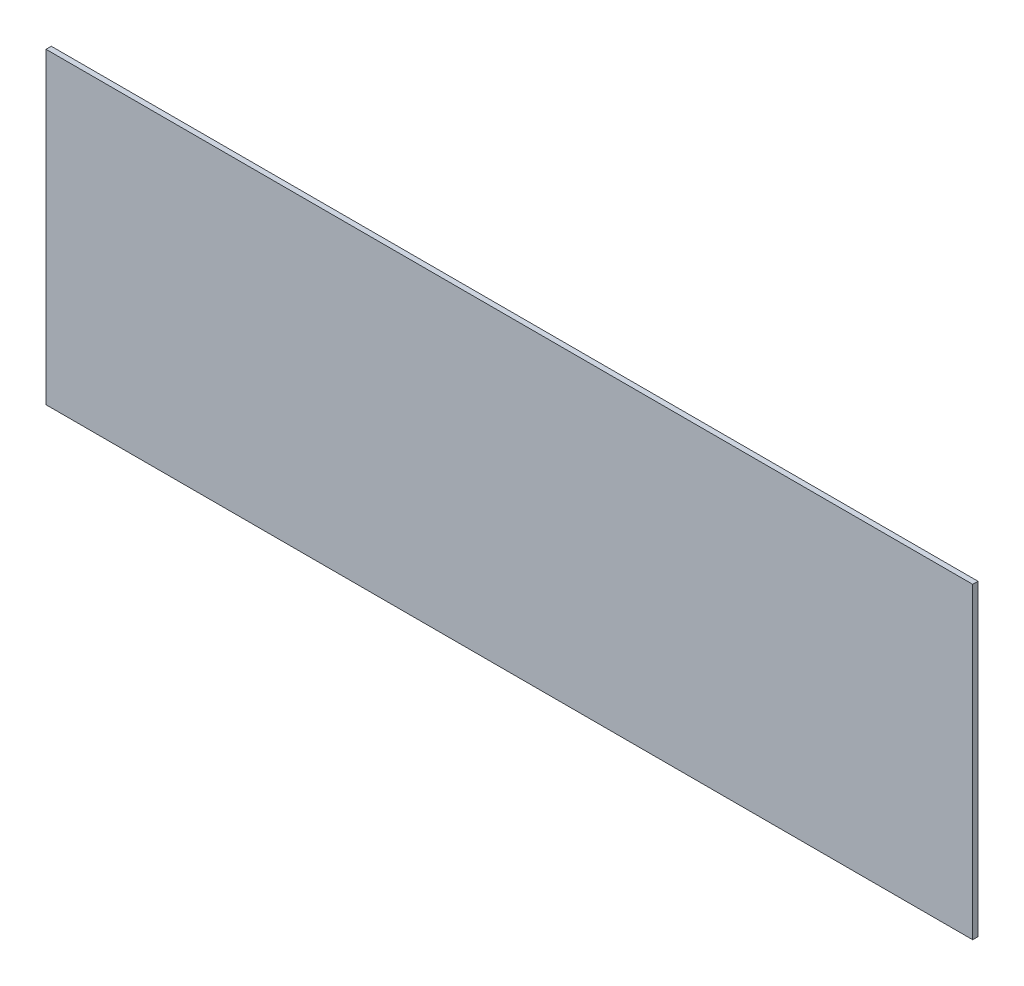
SolidWorks part; units mm, degrees
material "PMMA(有机玻璃)"
ref_plane "前视" through (0, 0, 0) normal (0, 0, 1) x (1, 0, 0)
ref_plane "上视" through (0, 0, 0) normal (0, 1, 0) x (1, 0, 0)
ref_plane "右视" through (0, 0, 0) normal (1, 0, 0) x (0, 0, -1)
sketch "草图1" plane through (0, 0, 0) normal (0, 0, 1) x (1, 0, 0)
  line L1 (-438, 145.5) -> (438, 145.5)
  line L2 (-438, 145.5) -> (-438, -145.5)
  line L3 (-438, -145.5) -> (438, -145.5)
  line L4 (438, 145.5) -> (438, -145.5)
  line L5 (-438, 145.5) -> (438, -145.5) construction
  line L6 (-438, -145.5) -> (438, 145.5) construction
  point P0 (0, 0)
  dimension "D1" = 291
  dimension "D2" = 876
extrude "凸台-拉伸1" add sketch "草图1" along normal blind 5
hole_wizard "M5 间隙孔1" positions "草图3" profile "草图2" hole size "M5" standard "GB"
sketch "草图3" plane through (0, 0, 5) normal (0, 0, 1) x (1, 0, 0)
  line L0 (-427.5, 273) -> (-427.5, -273) construction
  line L1 (-427.5, -273) -> (427.5, -273) construction
  line L2 (0, 273) -> (0, -273) construction
  line L3 (427.5, 273) -> (-427.5, 273) construction
  line L5 (-427.5, 0) -> (427.5, 0) construction
  line L6 (427.5, -273) -> (427.5, 273) construction
  point P0 (-375, -261)
  point P46 (415.5, 250)
  point P48 (-415.5, 250)
  point P58 (-125, -261)
  point P59 (125, -261)
  point P61 (-125, 261)
  point P62 (125, 261)
  point P64 (-375, 261)
  point P88 (375, -261)
  point P89 (375, 261)
  point P108 (415.5, 0)
  point P109 (-415.5, 0)
  point P110 (415.5, -250)
  point P111 (-415.5, -250)
  dimension "D1" = 12
  dimension "D2" = 12
  dimension "D5" = 3
  dimension "D3" = 12
  dimension "D6" = 4
  dimension "D4" = 2
sketch "草图2" plane through (-375, -261, 5) normal (1, 0, 0) x (0, -1, 0)
  line L0 (0, 0) -> (0, 5)
  line L1 (0, 5) -> (2.75, 5)
  line L2 (2.75, 5) -> (2.75, 0)
  line L5 (2.75, 0) -> (0, 0)
  line L11 (0, -6.35) -> (0, 107.95) construction
  dimension "通孔孔直径" = 5.5
  dimension "通孔孔深度" = 5
